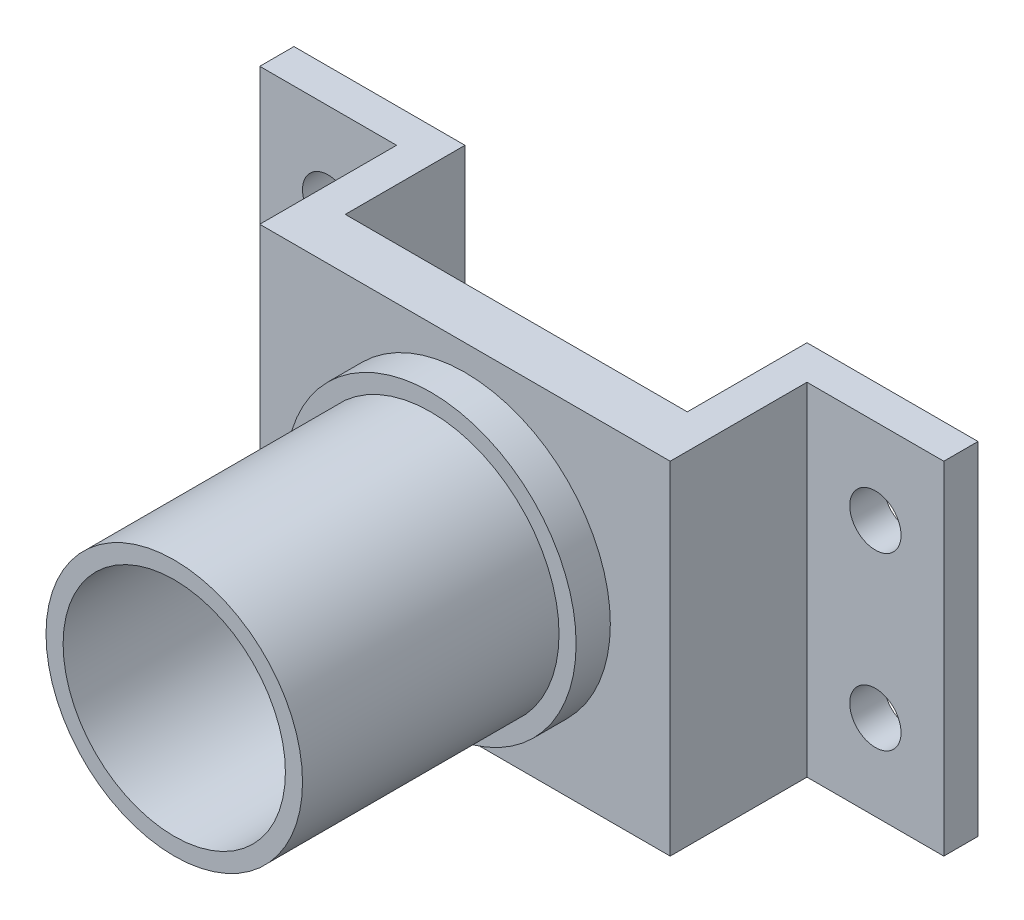
SolidWorks part; units mm, degrees
ref_plane "Front Plane" through (0, 0, 0) normal (0, 0, 1) x (1, 0, 0)
ref_plane "Top Plane" through (0, 0, 0) normal (0, 1, 0) x (1, 0, 0)
ref_plane "Right Plane" through (0, 0, 0) normal (1, 0, 0) x (0, 0, -1)
other "Configuration Table"
sketch "Sketch1" plane through (0, 0, 0) normal (0, 0, 1) x (1, 0, 0)
  circle A0 centre (0, 0) radius 6.5
  circle A1 centre (0, 0) radius 7.5
  dimension "D1" = 13
  dimension "D2" = 15
extrude "Boss-Extrude1" add sketch "Sketch1" along normal blind 22
ref_plane "Plane1" through (0, 0, 7) normal (0, 0, -1) x (-1, 0, 0)
sketch "Sketch2" plane through (0, 0, 7) normal (0, 0, -1) x (-1, 0, 0)
  circle A1 centre (0, 0) radius 7.5
  circle A2 centre (0, 0) radius 8.5
  dimension "D1" = 17
extrude "Boss-Extrude2" add sketch "Sketch2" along normal blind 2
sketch "Sketch5" plane through (0, 0, 0) normal (0, 0, -1) x (-1, 0, 0)
  circle A0 centre (0, 0) radius 6.5 construction
  circle A1 centre (0, 0) radius 7.5
  circle A2 centre (0, 0) radius 7.5
  circle A3 centre (0, 0) radius 6.5
  dimension "D1" = 0
extrude "Boss-Extrude4" add sketch "Sketch5" along normal blind 2
sketch "Sketch6" plane through (0, 0, -2) normal (0, 0, -1) x (-1, 0, 0)
  circle A0 centre (0, 0) radius 6.5 construction
  circle A1 centre (0, 0) radius 8.5
  circle A3 centre (0, 0) radius 6.5
extrude "Boss-Extrude5" add sketch "Sketch6" along normal blind 2
sketch "Sketch7" plane through (0, 0, 5) normal (0, 0, -1) x (-1, 0, 0)
  line L1 (15, -10) -> (-15, -10)
  line L2 (15, -10) -> (15, 10)
  line L3 (15, 10) -> (-15, 10)
  line L4 (-15, -10) -> (-15, 10)
  line L5 (0, 10) -> (0, -10) construction
  line L6 (15, 0) -> (-15, 0) construction
  point P0 (0, 0)
  dimension "D1" = 20
  dimension "D2" = 30
extrude "Boss-Extrude6" add sketch "Sketch7" along normal blind 10
sketch "Sketch8" plane through (0, -10, 0) normal (0, -1, 0) x (1, 0, 0)
  line L0 (15, -5) -> (-15, -5) construction
  line L1 (-10, -5) -> (10, -5)
  line L2 (-10, -5) -> (-10, 2)
  line L3 (-10, 2) -> (10, 2)
  line L4 (10, -5) -> (10, 2)
  line L5 (0, 0) -> (0, -5) construction
  point P9 (0, 2)
  dimension "D1" = 20
  dimension "D2" = 7
extrude "Cut-Extrude1" cut sketch "Sketch8" against normal through all
sketch "Sketch9" plane through (0, 0, -5) normal (0, 0, -1) x (-1, 0, 0)
  line L0 (-10, -10) -> (10, -10) construction
  line L1 (-15, 10) -> (-20, 10)
  line L2 (-15, 10) -> (-15, -10)
  line L3 (-15, -10) -> (-20, -10)
  line L4 (-20, 10) -> (-20, -10)
  line L5 (0, 15.372) -> (0, -21.5923) construction
  line L6 (20, 10) -> (20, -10)
  line L7 (15, -10) -> (20, -10)
  line L8 (15, 10) -> (15, -10)
  line L9 (15, 10) -> (20, 10)
  dimension "D1" = 5
extrude "Boss-Extrude7" add sketch "Sketch9" against normal blind 2
sketch "Sketch12" plane through (0, 0, 2) normal (0, 0, -1) x (-1, 0, 0)
  circle A0 centre (0, 0) radius 6.5
  dimension "D1" = 13
extrude "Cut-Extrude3" cut sketch "Sketch12" against normal through all
sketch "Sketch13" plane through (0, 0, 5) normal (0, 0, 1) x (1, 0, 0)
  line L0 (-15, 10) -> (-12, 10)
  line L1 (-15, 10) -> (15, 10) construction
  line L2 (-12, 10) -> (-12, -10)
  line L3 (15, -10) -> (-15, -10) construction
  line L4 (-12, -10) -> (-15, -10)
  line L5 (-15, -10) -> (-20, -10) construction
  line L6 (-15, -10) -> (-15, 10)
  line L7 (0, 12.9853) -> (0, -17.3753) construction
  line L8 (15, -10) -> (15, 10)
  line L9 (12, -10) -> (15, -10)
  line L10 (12, 10) -> (12, -10)
  line L11 (15, 10) -> (12, 10)
  dimension "D1" = 3
extrude "Cut-Extrude4" cut sketch "Sketch13" against normal blind 8
sketch "Sketch11" plane through (0, 0, -3) normal (0, 0, 1) x (1, 0, 0)
  line L0 (16, 10) -> (16, -10) construction
  line L1 (12, 10) -> (20, 10) construction
  line L2 (20, -10) -> (12, -10) construction
  line L3 (0, 0) -> (0, 16.5236) construction
  line L4 (-16, 10) -> (-16, -10) construction
  circle A0 centre (16, 5) radius 1.5
  circle A1 centre (16, -5) radius 1.5
  circle A2 centre (-16, -5) radius 1.5
  circle A3 centre (-16, 5) radius 1.5
  dimension "D1" = 3
  dimension "D2" = 5
  dimension "D3" = 10
extrude "Cut-Extrude2" cut sketch "Sketch11" against normal through all
